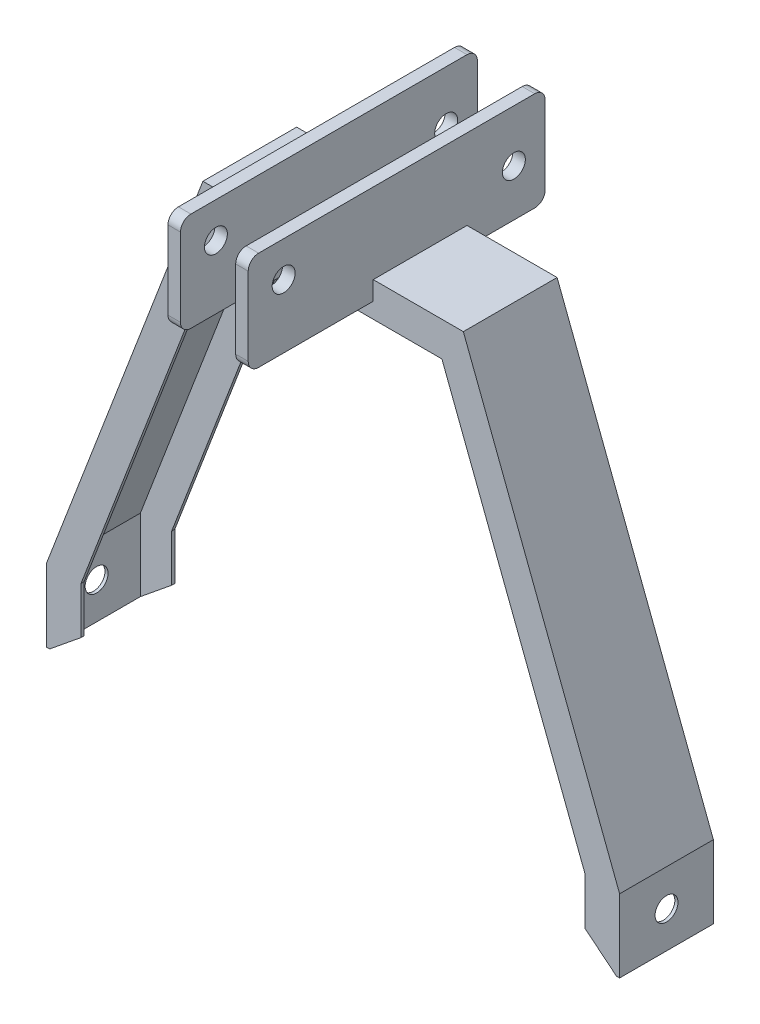
from build123d import *

# Parameters (mm, degrees)
SHEET_EXTRUDE_1_1_BACK   = 45
SHEET_EXTRUDE_1_1_DEPTH  = 90
THICKEN_1_T2             = 3
EXTRUDE_START            = 42
EXTRUDE_3_DEPTH          = 3
CUT_EXTRUDE_1_DEPTH      = 811.963488807
CUT_EXTRUDE_1_DEPTH_BACK = 811.963488807
SKETCH_4_R               = 11
EXTRUDE_START_2          = 26.5
SKETCH_5_R               = 11
EXTRUDE_4_DEPTH          = 12


with BuildPart() as body_1:
    # Sheet Extrude 1: a surface, the sketch's curves swept straight by 90 mm
    with BuildLine(Plane.XY.offset(489.577688539).offset(-SHEET_EXTRUDE_1_1_BACK), mode=Mode.PRIVATE) as sheet_extrude_1_1_path:
        Line((-1467.361703007, 82), (-1467.361703007, 152))
        Line((-1467.361703007, 152), (-1317.361703007, 544.300904919))
        Line((-1317.361703007, 544.300904919), (-1067.361703007, 544.300904919))
        Line((-1067.361703007, 544.300904919), (-917.361703007, 152))
        Line((-917.361703007, 152), (-917.361703007, 82))
    sheet_extrude_1_1 = Shell.extrude(sheet_extrude_1_1_path.wire(), (0 * SHEET_EXTRUDE_1_1_DEPTH, 0 * SHEET_EXTRUDE_1_1_DEPTH, 1 * SHEET_EXTRUDE_1_1_DEPTH))
    add(Solid.thicken(sheet_extrude_1_1, -THICKEN_1_T2))

    # 草图3 → 凸台-拉伸3 (add)
    with BuildSketch(Plane.XY.offset(489.577688539).offset(EXTRUDE_START)):
        Polygon((-1464.361703007, 82), (-1434.361703007, 106.446018098), (-1434.361703007, 151.446018098), (-1296.767748095, 511.300904919), (-1192.361703007, 511.300904919), (-1192.361703007, 541.300904919), (-1315.296961402, 541.300904919), (-1464.361703007, 151.446018098), align=None)
    extrude(amount=EXTRUDE_3_DEPTH)

    # 镜向1: body 1 across plane


with BuildPart() as body_1_1:
    add(body_1.part)
    add(body_1.part.mirror(Plane.ZY.offset(1192.361703007)))

    # 镜向2: body 1 across plane


with BuildPart() as body_1_2:
    add(body_1_1.part)
    add(body_1_1.part.mirror(Plane.XY.offset(489.577688539)))

    # 草图4 → 切除-拉伸1 (cut, two sides: drawn at the far end of the back side and taken through both)
    with BuildSketch(Plane.ZY.offset(1192.361703007).offset(-CUT_EXTRUDE_1_DEPTH_BACK)):
        with Locations((489.577688539, 117)):
            Circle(SKETCH_4_R)
    extrude(amount=CUT_EXTRUDE_1_DEPTH + CUT_EXTRUDE_1_DEPTH_BACK, mode=Mode.SUBTRACT)

    # 草图5 → 凸台-拉伸4 (add)
    with BuildSketch(Plane.ZY.offset(1192.361703007).offset(EXTRUDE_START_2)):
        with BuildLine():
            Line((379.577688539, 621.300904919), (644.577688539, 621.300904919))
            ThreePointArc((644.577688539, 621.300904919), (651.64875635, 618.371972731), (654.577688539, 611.300904919))
            Line((654.577688539, 611.300904919), (654.577688539, 536.300904919))
            ThreePointArc((654.577688539, 536.300904919), (651.64875635, 529.229837107), (644.577688539, 526.300904919))
            Line((644.577688539, 526.300904919), (379.577688539, 526.300904919))
            ThreePointArc((379.577688539, 526.300904919), (372.506620727, 529.229837107), (369.577688539, 536.300904919))
            Line((369.577688539, 536.300904919), (369.577688539, 611.300904919))
            ThreePointArc((369.577688539, 611.300904919), (372.506620727, 618.371972731), (379.577688539, 621.300904919))
        make_face()
        with Locations((620.577688539, 587.300904919)):
            Circle(SKETCH_5_R, mode=Mode.SUBTRACT)
        with Locations((399.577688539, 571.300904919)):
            Circle(SKETCH_5_R, mode=Mode.SUBTRACT)
    extrude(amount=EXTRUDE_4_DEPTH)

    # 镜向3: body 1 across plane


with BuildPart() as body_1_3:
    add(body_1_2.part)
    add(body_1_2.part.mirror(Plane.ZY.offset(1192.361703007)))


solid = body_1_3.part
